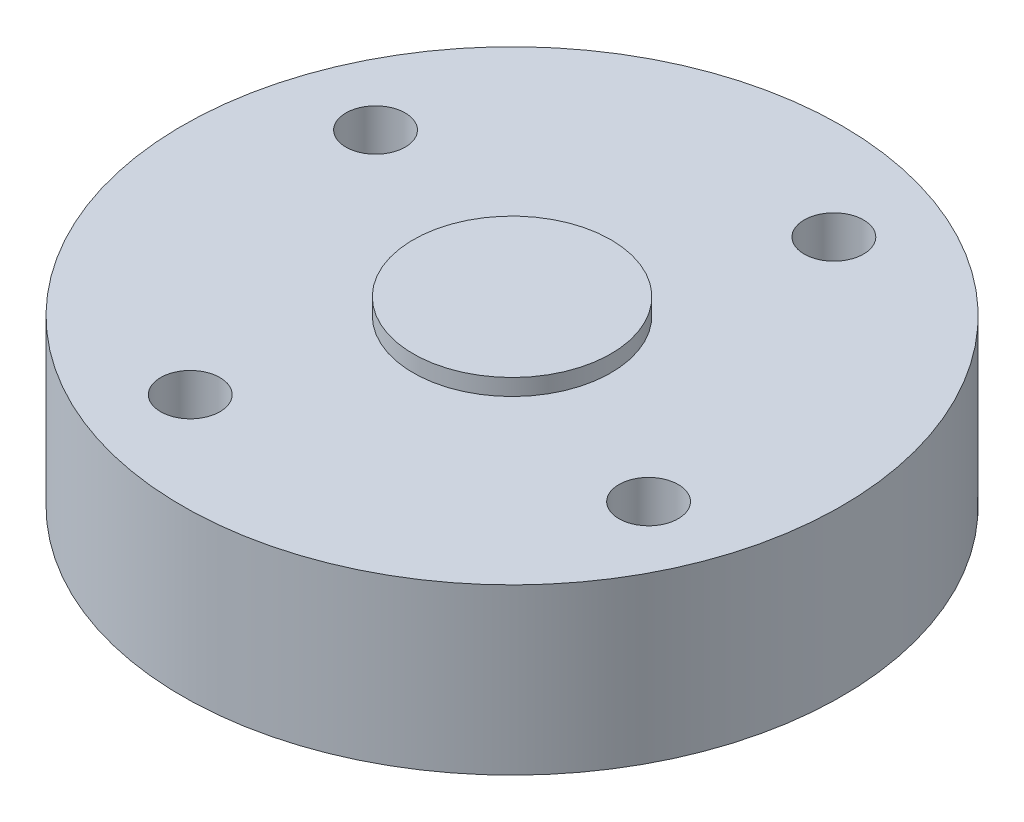
SolidWorks part; units mm, degrees
material "AISI 1045 钢，冷拔"
ref_plane "Front Plane" through (0, 0, 0) normal (0, 0, 1) x (1, 0, 0)
ref_plane "Top Plane" through (0, 0, 0) normal (0, 1, 0) x (1, 0, 0)
ref_plane "Right Plane" through (0, 0, 0) normal (1, 0, 0) x (0, 0, -1)
sketch "Sketch1" plane through (0, 0, 0) normal (0, 0, 1) x (1, 0, 0)
  line L0 (58.9461, 0) -> (0, 0) construction
  line L1 (0, 0) -> (0, 89.3907) construction
  line L2 (30, -31.6) -> (100, -31.6)
  line L4 (30, -31.6) -> (30, -26.6)
  line L5 (30, -26.6) -> (0, -26.6)
  line L9 (100, -31.6) -> (100, -81.6)
  line L10 (100, -81.6) -> (25, -81.6)
  line L11 (25, -81.6) -> (25, -121.6)
  line L12 (25, -121.6) -> (0, -121.6)
  line L13 (0, -121.6) -> (0, -26.6)
  point P3 (80.4, 0)
  dimension "D1" = 5
  dimension "D2" = 60
  dimension "D3" = 200
  dimension "D4" = 50
  dimension "D5" = 50
  dimension "D6" = 40
revolve "Revolve1" add sketch "Sketch1" angle 360 about L1
chamfer "Chamfer2" [suppressed] distance 0.5 angle 45
hole_wizard "Ø18.0 (18) Diameter Hole1" positions "Sketch5" profile "Sketch4" hole size "Ø18.0" standard "GB"
sketch "Sketch5" plane through (0, -31.6, 0) normal (0, 1, 0) x (1, 0, 0)
  circle A0 centre (-69.5333, 28.109) radius 7 construction
  circle A1 centre (-28.109, -69.5333) radius 7 construction
  circle A2 centre (69.5333, -28.109) radius 7 construction
  circle A3 centre (28.109, 69.5333) radius 7 construction
  point P1 (-69.5333, 28.109)
  point P6 (-28.109, -69.5333)
  point P11 (69.5333, -28.109)
  point P16 (28.109, 69.5333)
sketch "Sketch4" plane through (-69.5333, -31.6, -28.109) normal (1, 0, 0) x (0, 0, 1)
  line L0 (0, 0) -> (0, 90)
  line L1 (0, 90) -> (9, 90)
  line L2 (9, 90) -> (9, 0)
  line L5 (9, 0) -> (0, 0)
  line L11 (0, -6.35) -> (0, 107.95) construction
  dimension "通孔孔直径" = 18
  dimension "通孔孔深度" = 90
